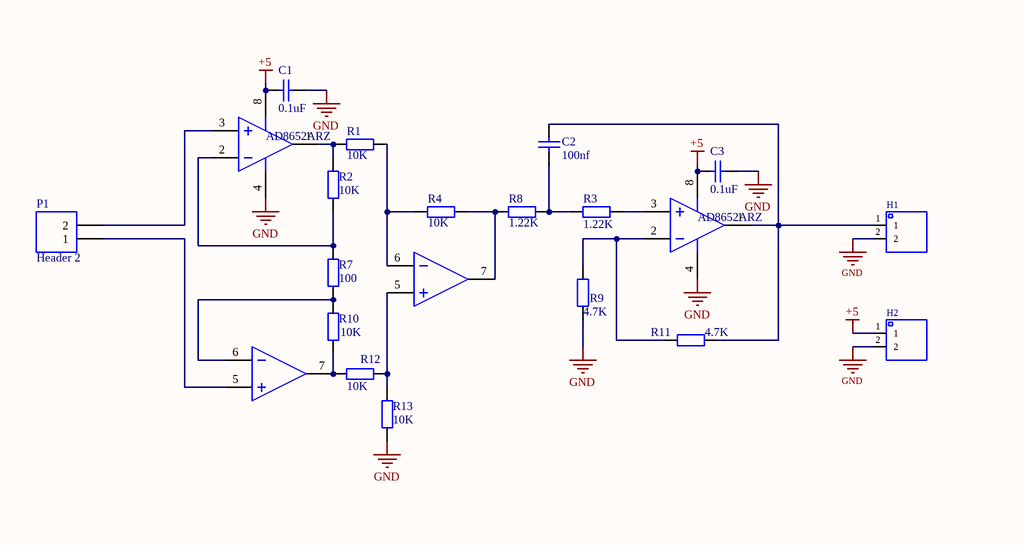
[diagram p0: MISC49864-3.schdoc, left]
# Altium project MISC49864-2.PrjPcb
1 sheet, 19 parts. Net scope: global (net labels, ports and power ports of the same name join across sheets).
Board file: MISC49864.pcbdoc

## Sheet MISC49864-3.schdoc
size 566 x 399 mm; DocumentNumber: MISC49864; SheetNumber: 1; SheetTotal: 1; Name: MISC49864

### Parts
C1  value 0.1uF  [CAP-TH_L5.0-W2.5-P5.00-D1.0]  (hidden comment: Cap)
C2  value 100nf  [CAP-TH_L5.0-W2.5-P5.00-D1.0]  (hidden comment: Cap)
C3  value 0.1uF  [CAP-TH_L5.0-W2.5-P5.00-D1.0]  (hidden comment: Cap)
H1  (no value)  [HDR-TH_2P-P2.54-V-M-1]
H2  (no value)  [HDR-TH_2P-P2.54-V-M-1]
P1  Header 2  [HDR-TH_2P-P2.54-V-M-1]
R1  10K  [R0603_SMD-CRCW060327R0FKEA]
R2  10K  [R0603_SMD-CRCW060327R0FKEA]
R3  1.22K  [R0603_SMD-CRCW060327R0FKEA]
R4  10K  [R0603_SMD-CRCW060327R0FKEA]
R7  100  [R0603_SMD-CRCW060327R0FKEA]
R8  1.22K  [R0603_SMD-CRCW060327R0FKEA]
R9  4.7K  [R0603_SMD-CRCW060327R0FKEA]
R10  10K  [R0603_SMD-CRCW060327R0FKEA]
R11  4.7K  [R0603_SMD-CRCW060327R0FKEA]
R12  10K  [R0603_SMD-CRCW060327R0FKEA]
R13  10K  [R0603_SMD-CRCW060327R0FKEA]
U1  AD8652ARZ  [SOIC-8_L4.9-W3.9-P1.27-LS6.0-BL]  (parts A,B of 2)
U2  AD8652ARZ  [SOIC-8_L4.9-W3.9-P1.27-LS6.0-BL]  (parts A,B of 2)

### Nets
+5: C1.1 C3.1 H2.1 U1.8(V+) U2.8(V+)
GND: C1.2 C3.2 H1.2 H2.2 R9.1 R13.2 U1.4(V-) U2.4(V-)
NetC2_1: C2.1 H1.1 R11.2 U2.1(OUTA)
NetC2_2: C2.2 R3.1 R8.2
NetP1_1: P1.1 U1.5(+INB)
NetP1_2: P1.2 U1.3(+INA)
NetR1_1: R1.1 R4.2 U2.6(-INB)
NetR1_2: R1.2 R2.2 U1.1(OUTA)
NetR2_1: R2.1 R7.2 U1.2(-INA)
NetR3_2: R3.2 U2.3(+INA)
NetR4_1: R4.1 R8.1 U2.7(OUTB)
NetR7_1: R7.1 R10.2 U1.6(-INB)
NetR9_2: R9.2 R11.1 U2.2(-INA)
NetR10_1: R10.1 R12.2 U1.7(OUTB)
NetR12_1: R12.1 R13.1 U2.5(+INB)

### Library data of the parts
C1 = Cap: Capacitor; Origin Footprint: 0805; UniqueId: 5fb4f22ffcb6a001; AddInBom: yes; Device: Cap; Published: 8-Jun-2000; LatestRevisionDate: 17-Jul-2002; LatestRevisionNote: Re-released for DXP Platform.; PackageReference: RAD-0.3; PackageDescription: Radial Cap, Thru-Hole; 2 Leads; 0.3 in Pin Spacing; DesignItemID: Cap; LibraryName: AD1; SymbolName: Cap; Publisher: Altium Limited
C2 = Cap: Capacitor; Origin Footprint: 0805; UniqueId: 21d50210554cb61f; AddInBom: yes; Device: Cap; Published: 8-Jun-2000; LatestRevisionDate: 17-Jul-2002; LatestRevisionNote: Re-released for DXP Platform.; PackageReference: RAD-0.3; PackageDescription: Radial Cap, Thru-Hole; 2 Leads; 0.3 in Pin Spacing; DesignItemID: Cap; LibraryName: AD1; SymbolName: Cap; Publisher: Altium Limited
C3 = Cap: Capacitor; Origin Footprint: 0805; UniqueId: ec64484c8c07847f; AddInBom: yes; Device: Cap; Published: 8-Jun-2000; LatestRevisionDate: 17-Jul-2002; LatestRevisionNote: Re-released for DXP Platform.; PackageReference: RAD-0.3; PackageDescription: Radial Cap, Thru-Hole; 2 Leads; 0.3 in Pin Spacing; DesignItemID: Cap; LibraryName: AD1; SymbolName: Cap; Publisher: Altium Limited
H1 H2 = HDR-M_2.54_1x2P: Symbol: 210S-1*2P L=11.6MMGold-plated black; ConvertToPcb: yes; ModelId: 79b2e9f2d70a4d68a1b7098f27c6d4c50819f05c4eef4c71ace90d822a990e87; ModelName: HDR-M-2.54_1x2; ModelTransform: 200,100,0,0,0,0,0,0,-118.11; Device: HDR-M_2.54_1x2P; AddInBom: yes; SupplierPart: C124375; Supplier Footprint: 插件; FootprintName: HDR-TH_2P-P2.54-V-M-1
P1 = Header 2: Header, 2-Pin; Origin Footprint: HDR1X2; UniqueId: f88e3064cb77b82c; AddInBom: yes; Device: Header 2; LatestRevisionDate: 17-Jul-2002; LatestRevisionNote: Re-released for DXP Platform.; DesignItemID: Header 2; LibraryName: Miscellaneous Connectors; SymbolName: Header 2; Publisher: Altium Limited
R1 = 10K_1: Resistor; Value: RMK1608MB472JM; CommValue: 4.7kΩ; Origin Footprint: 0805; UniqueId: 4e166b190d4de1c3; SymbolName: Res0805; AddInBom: yes; Device: 10K_1; Published: 2014-3-10; LatestRevisionDate: 2014-3-10; LatestRevisionNote: AD10; PackageDescription: SR; Materi: Resistor; DesignItemID: Res0805; LibraryName: strain_gage; Publisher: SAST_HZ
R2 = 10K: Resistor; Value: RMK1608MB472JM; CommValue: 4.7kΩ; Origin Footprint: 0805; UniqueId: 06442d24ab060343; SymbolName: Res0805; AddInBom: yes; Device: 10K; Published: 2014-3-10; LatestRevisionDate: 2014-3-10; LatestRevisionNote: AD10; PackageDescription: SR; Materi: Resistor; DesignItemID: Res0805; LibraryName: strain_gage; Publisher: SAST_HZ
R3 = 1.22K: Resistor; Origin Footprint: 0805; UniqueId: 6e26aea592918673; SymbolName: Res2; AddInBom: yes; Device: 1.22K; Published: 8-Jun-2000; LatestRevisionDate: 17-Jul-2002; LatestRevisionNote: Re-released for DXP Platform.; PackageReference: AXIAL-0.4; PackageDescription: Axial Device, Thru-Hole; 2 Leads; 0.4 in Pin Spacing; DesignItemID: Res2; LibraryName: AD1; Publisher: Altium Limited
R4 = 10K_1: Resistor; Value: RMK1608MB472JM; CommValue: 4.7kΩ; Origin Footprint: 0805; UniqueId: 49359f7360e76581; SymbolName: Res0805; AddInBom: yes; Device: 10K_1; Published: 2014-3-10; LatestRevisionDate: 2014-3-10; LatestRevisionNote: AD10; PackageDescription: SR; Materi: Resistor; DesignItemID: Res0805; LibraryName: strain_gage; Publisher: SAST_HZ
R7 = 100: Resistor; Value: RMK1608MB472JM; CommValue: 4.7kΩ; Origin Footprint: 0805; UniqueId: 01f5c70ff2630ee7; SymbolName: Res0805; AddInBom: yes; Device: 100; Published: 2014-3-10; LatestRevisionDate: 2014-3-10; LatestRevisionNote: AD10; PackageDescription: SR; Materi: Resistor; DesignItemID: Res0805; LibraryName: strain_gage; Publisher: SAST_HZ
R8 = 1.22K: Resistor; Origin Footprint: 0805; UniqueId: f0665cc51e401020; SymbolName: Res2; AddInBom: yes; Device: 1.22K; Published: 8-Jun-2000; LatestRevisionDate: 17-Jul-2002; LatestRevisionNote: Re-released for DXP Platform.; PackageReference: AXIAL-0.4; PackageDescription: Axial Device, Thru-Hole; 2 Leads; 0.4 in Pin Spacing; DesignItemID: Res2; LibraryName: AD1; Publisher: Altium Limited
R9 = 4.7K: Resistor; Value: RMK1608MB472JM; CommValue: 4.7kΩ; Origin Footprint: 0805; UniqueId: 7a9d276dcc23a651; SymbolName: Res0805; AddInBom: yes; Device: 4.7K; Published: 2014-3-10; LatestRevisionDate: 2014-3-10; LatestRevisionNote: AD10; PackageDescription: SR; Materi: Resistor; DesignItemID: Res0805; LibraryName: strain_gage; Publisher: SAST_HZ
R10 = 10K: Resistor; Value: RMK1608MB472JM; CommValue: 4.7kΩ; Origin Footprint: 0805; UniqueId: 7663007c1f2bc029; SymbolName: Res0805; AddInBom: yes; Device: 10K; Published: 2014-3-10; LatestRevisionDate: 2014-3-10; LatestRevisionNote: AD10; PackageDescription: SR; Materi: Resistor; DesignItemID: Res0805; LibraryName: strain_gage; Publisher: SAST_HZ
R11 = 4.7K_1: Resistor; Value: RMK1608MB472JM; CommValue: 4.7kΩ; Origin Footprint: 0805; UniqueId: 069ba0dc55a84bc8; SymbolName: Res0805; AddInBom: yes; Device: 4.7K_1; Published: 2014-3-10; LatestRevisionDate: 2014-3-10; LatestRevisionNote: AD10; PackageDescription: SR; Materi: Resistor; DesignItemID: Res0805; LibraryName: strain_gage; Publisher: SAST_HZ
R12 = 10K_1: Resistor; Value: RMK1608MB472JM; CommValue: 4.7kΩ; Origin Footprint: 0805; UniqueId: f574a6082c36e6cb; SymbolName: Res0805; AddInBom: yes; Device: 10K_1; Published: 2014-3-10; LatestRevisionDate: 2014-3-10; LatestRevisionNote: AD10; PackageDescription: SR; Materi: Resistor; DesignItemID: Res0805; LibraryName: strain_gage; Publisher: SAST_HZ
R13 = 10K: Resistor; Value: RMK1608MB472JM; CommValue: 4.7kΩ; Origin Footprint: 0805; UniqueId: ff7631ddbc1e2fda; SymbolName: Res0805; AddInBom: yes; Device: 10K; Published: 2014-3-10; LatestRevisionDate: 2014-3-10; LatestRevisionNote: AD10; PackageDescription: SR; Materi: Resistor; DesignItemID: Res0805; LibraryName: strain_gage; Publisher: SAST_HZ
U1 = AD8652ARZ: Manufact: ADI/LINEAR; Add into BOM: yes; Number of Circuits: 2; Gain Bandwidth Product(GBP): 50MHz; Slew Rate(SR): 41V/us; UniqueId: 48a4a086d8c42a18; Device: AD8652ARZ; LCSC Part Name: AD8652ARZ; Supplier Part: C207966; Manufacturer Part: AD8652ARZ; Supplier Footprint: SOIC-8; JLCPCB Part Class: Extended Part; Datasheet: https://atta.szlcsc.com/upload/public/pdf/source/20180424/C207966_515245321259DBE42786E38615D37704.pdf; Supplier: LCSC; Convert to PCB: yes; DesignItemID: AD8652ARZ; LibraryName: strain_gage; SymbolName: AD8652ARZ; FootprintName: SOIC-8_L4.9-W3.9-P1.27-LS6.0-BL
U2 = AD8652ARZ: Manufact: ADI/LINEAR; Add into BOM: yes; Number of Circuits: 2; Gain Bandwidth Product(GBP): 50MHz; Slew Rate(SR): 41V/us; UniqueId: d74c11912b695046; Device: AD8652ARZ; LCSC Part Name: AD8652ARZ; Supplier Part: C207966; Manufacturer Part: AD8652ARZ; Supplier Footprint: SOIC-8; JLCPCB Part Class: Extended Part; Datasheet: https://atta.szlcsc.com/upload/public/pdf/source/20180424/C207966_515245321259DBE42786E38615D37704.pdf; Supplier: LCSC; Convert to PCB: yes; DesignItemID: AD8652ARZ; LibraryName: strain_gage; SymbolName: AD8652ARZ; FootprintName: SOIC-8_L4.9-W3.9-P1.27-LS6.0-BL